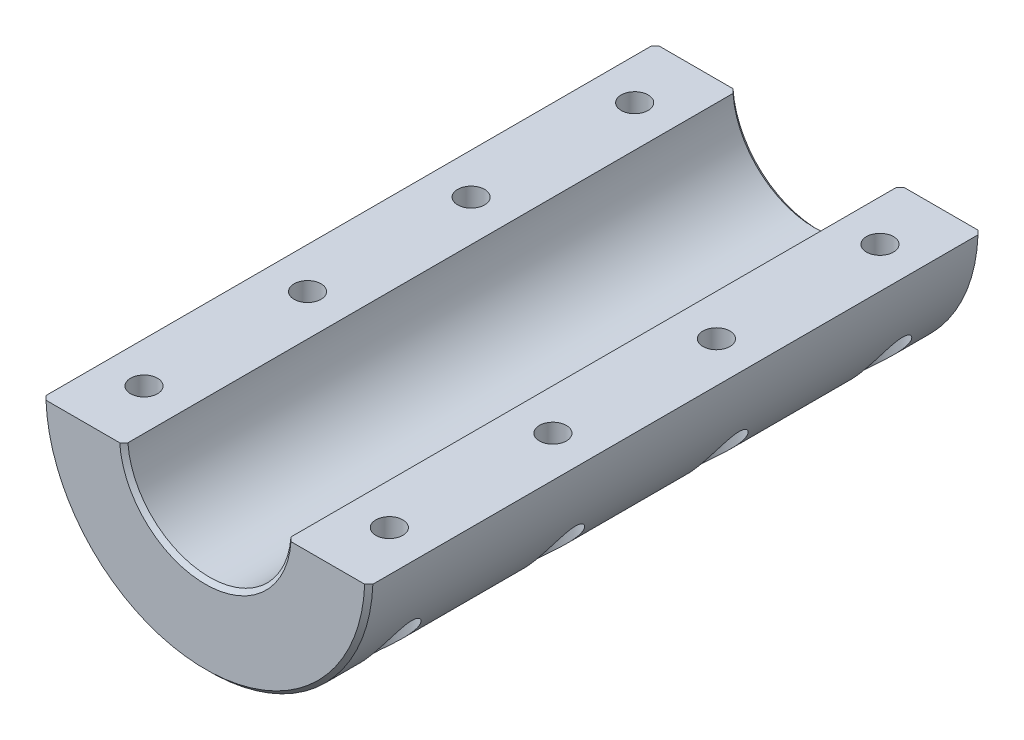
SolidWorks part; units mm, degrees
material "Plain carbon steel"
ref_plane "Front Plane" through (0, 0, 0) normal (0, 0, 1) x (1, 0, 0)
ref_plane "Top Plane" through (0, 0, 0) normal (0, 1, 0) x (1, 0, 0)
ref_plane "Right Plane" through (0, 0, 0) normal (1, 0, 0) x (0, 0, -1)
sketch "Sketch1" plane through (0, 0, 0) normal (0, 0, 1) x (1, 0, 0)
  line L0 (0, 15.3) -> (0, 0) construction
  line L1 (-4, 15.3) -> (4, 15.3)
  line L2 (-4, 15.3) -> (-4, 19.5959)
  line L4 (4, 15.3) -> (4, 19.5959)
  arc A0 (-4, 19.5959) -> (4, 19.5959) centre (0, 0) ccw
  circle A1 centre (0, 0) radius 40
  dimension "D1" = 40
  dimension "D2" = 80
  dimension "D4" = 15.3
  dimension "D3" = 8
extrude "Boss-Extrude1" add sketch "Sketch1" along normal mid plane 150
chamfer "Chamfer1" distance 1 angle 45 4 edges at (0, -20, 75) (40, 0, 75) (0, -20, -75) (40, 0, -75)
sketch "Sketch2" plane through (0, 0, 75) normal (0, 0, 1) x (1, 0, 0)
  line L1 (-42.5, 1.5) -> (42.5, 1.5)
  line L2 (-42.5, 1.5) -> (-42.5, -1.5)
  line L3 (-42.5, -1.5) -> (42.5, -1.5)
  line L4 (42.5, 1.5) -> (42.5, -1.5)
  line L5 (-42.5, 1.5) -> (42.5, -1.5) construction
  line L6 (-42.5, -1.5) -> (42.5, 1.5) construction
  point P0 (0, 0)
  dimension "D1" = 3
  dimension "D2" = 85
extrude "Cut-Extrude1" cut sketch "Sketch2" against normal blind 180
hole_wizard "M6 Clearance Hole1" positions "Sketch4" profile "Sketch5" hole size "M6" standard "GB"
sketch "Sketch4" plane through (0, -1.5, 0) normal (0, -1, 0) x (-1, 0, 0)
  point P0 (-30, -60)
  dimension "D1" = 60
  dimension "D2" = 30
sketch "Sketch5" plane through (30, -1.5, 60) normal (1, 0, 0) x (0, 0, 1)
  line L0 (0, 0) -> (0, 36.9828)
  line L1 (0, 36.9828) -> (3.3, 35)
  line L2 (3.3, 35) -> (3.3, 0)
  line L5 (3.3, 0) -> (0, 0)
  line L10 (0, 36.9828) -> (-3.3, 35) construction
  line L11 (0, -6.35) -> (0, 107.95) construction
  dimension "孔直径" = 6.6
  dimension "孔深度" = 35
  dimension "导头角度" = 118
sketch "Sketch6" plane through (0, -1.5, 0) normal (0, 1, 0) x (1, 0, 0)
  circle A0 centre (30, -60) radius 5.5
  dimension "D1" = 11
extrude "Cut-Extrude2" cut sketch "Sketch6" against normal blind 91 from offset 9 offset against normal yes
pattern_linear "LPattern1" count 4 spacing 40 along (0, 0, -1) count 2 spacing 60 along (-1, 0, 0) of "M6 Clearance Hole1", "Cut-Extrude2"
